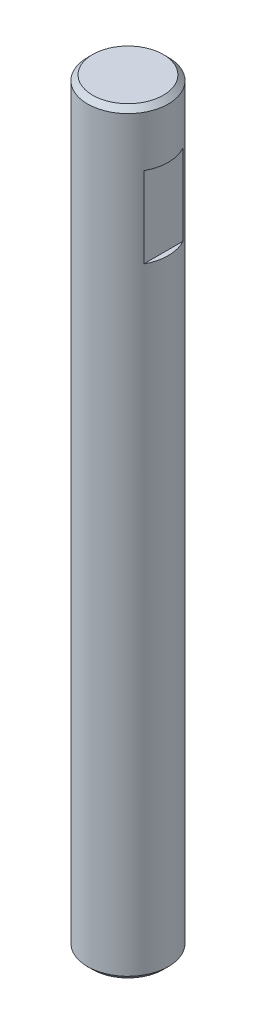
SolidWorks part; units mm, degrees
ref_plane "Front Plane" through (0, 0, 0) normal (0, 0, 1) x (1, 0, 0)
ref_plane "Top Plane" through (0, 0, 0) normal (0, 1, 0) x (1, 0, 0)
ref_plane "Right Plane" through (0, 0, 0) normal (1, 0, 0) x (0, 0, -1)
sketch "Sketch1" plane through (0, 0, 0) normal (0, 1, 0) x (1, 0, 0)
  circle A0 centre (0, 0) radius 4
  dimension "D1" = 8
extrude "Boss-Extrude1" add sketch "Sketch1" along normal blind 75
chamfer "Chamfer1" distance 0.5 angle 45 2 edges at (0, 0, 4) (0, 75, 4)
sketch "Sketch2" plane through (0, 0, 0) normal (0, 0, 1) x (1, 0, 0)
  line L0 (0, 0) -> (0, 50000) construction
  line L1 (4, 0.5) -> (4, 74.5) construction
  line L2 (3.5, 69.5) -> (4.5, 69.5)
  line L3 (3.5, 69.5) -> (3.5, 61.5)
  line L4 (3.5, 61.5) -> (4.5, 61.5)
  line L5 (4.5, 69.5) -> (4.5, 61.5)
  line L6 (3.5, 69.5) -> (4.5, 61.5) construction
  line L7 (3.5, 61.5) -> (4.5, 69.5) construction
  line L8 (3.5, 75) -> (-3.5, 75) construction
  point P3 (4, 65.5)
  dimension "D1" = 9.5
  dimension "D2" = 3.5
  dimension "D3" = 8
extrude "Cut-Extrude1" cut sketch "Sketch2" against normal mid plane 10
